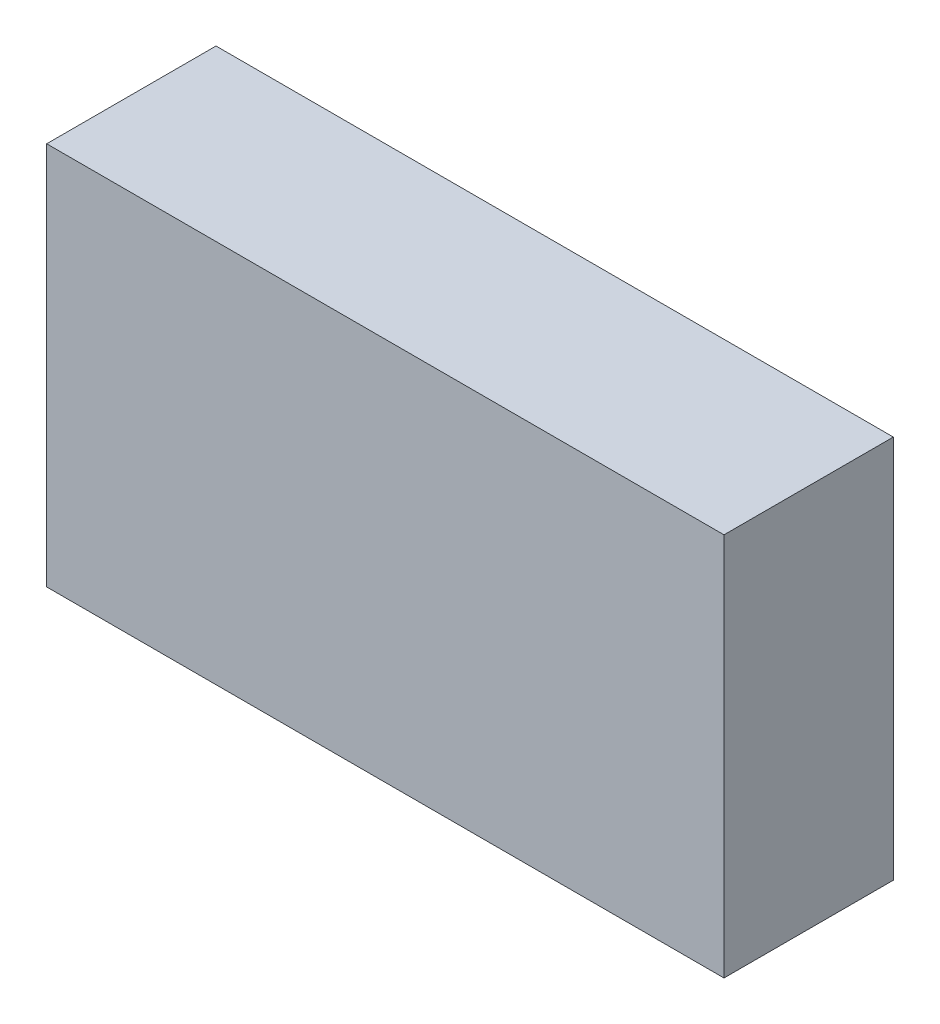
SolidWorks part; units mm, degrees
material "6061 合金"
ref_plane "前视基准面" through (0, 0, 0) normal (0, 0, 1) x (1, 0, 0)
ref_plane "上视基准面" through (0, 0, 0) normal (0, 1, 0) x (1, 0, 0)
ref_plane "右视基准面" through (0, 0, 0) normal (1, 0, 0) x (0, 0, -1)
sketch "草图1" plane through (0, 0, 0) normal (0, 0, 1) x (1, 0, 0)
  line L1 (30, -17) -> (-30, -17)
  line L2 (30, -17) -> (30, 17)
  line L3 (30, 17) -> (-30, 17)
  line L4 (-30, -17) -> (-30, 17)
  line L5 (30, -17) -> (-30, 17) construction
  line L6 (30, 17) -> (-30, -17) construction
  point P0 (0, 0)
  dimension "D1" = 60
  dimension "D2" = 34
extrude "凸台-拉伸1" add sketch "草图1" along normal blind 15
